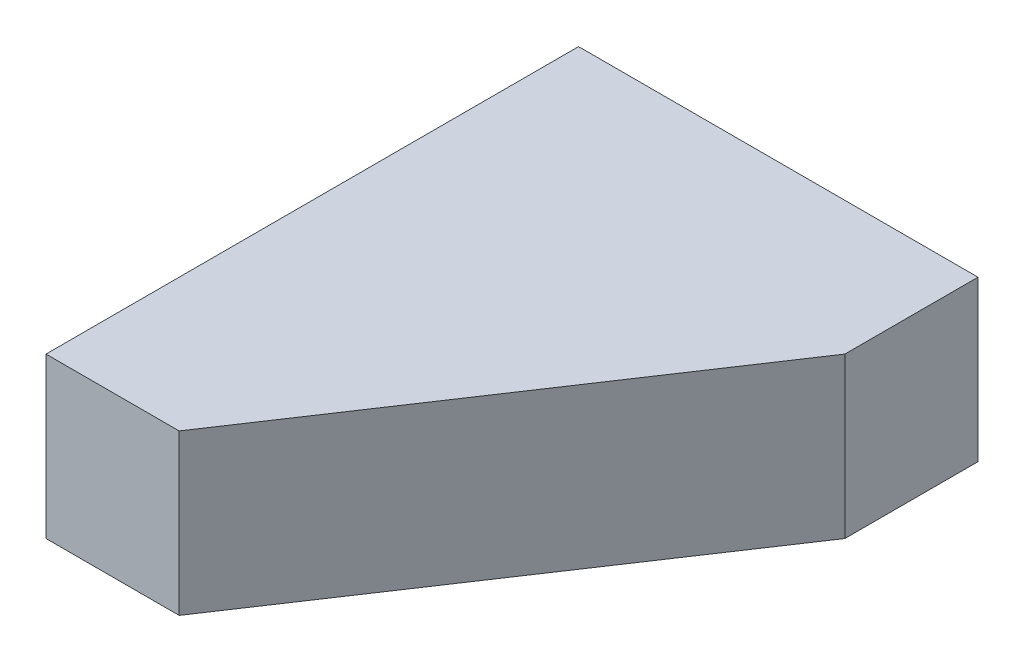
from build123d import *

# Parameters (mm, degrees)
EXTRUDE1_DEPTH = 6


with BuildPart() as part:
    # Sketch1 → Extrude1 (new, symmetric)
    with BuildSketch(Plane(origin=(0, 0, 0), x_dir=(1, 0, 0), z_dir=(0, 1, 0))):
        Polygon((-15, -20), (-5, -20), (15, 10), (15, 20), (-15, 20), align=None)
    extrude(amount=EXTRUDE1_DEPTH, both=True)


solid = part.part
